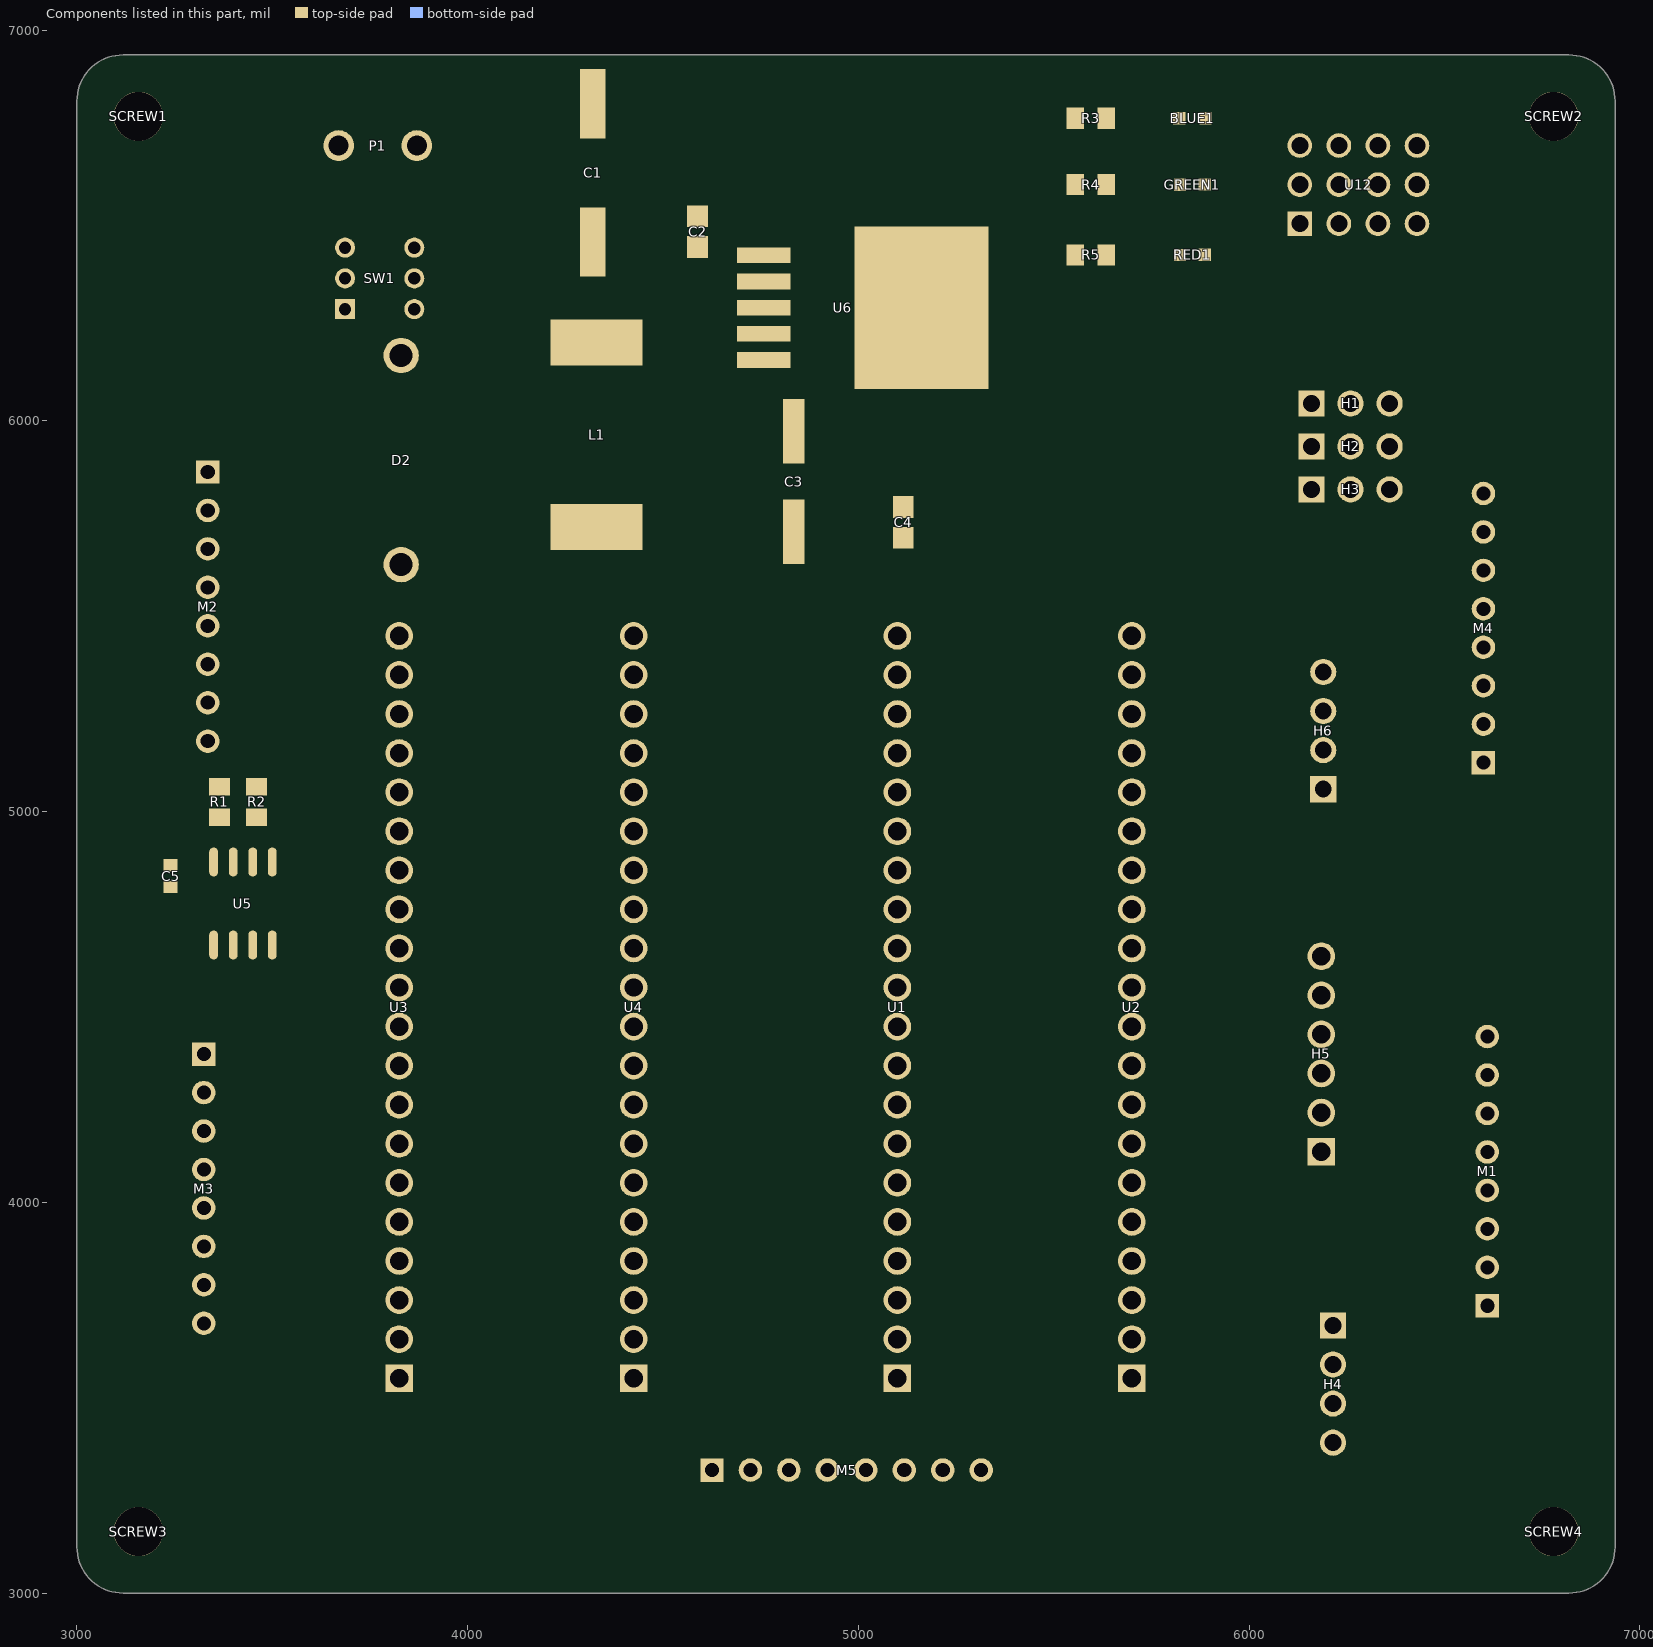
[diagram p0: the components of this part, seen from the top]
# Altium PCB MISC50151.pcbdoc (part 4 of 4)
Units mil, origin at the board's own origin, x right, y up, seen from the top; angles counter-clockwise.
Board outline 3937.01 x 3937.01 mil, 4 copper layers (Top Layer, Inner1, Inner2, Bottom Layer), stack 62.447 mil thick; 39 components, 26 nets, 211 pads, 230 vias.

## Other copper (continued)
Bottom Layer:
  region net M_PWM1: 6324.25,6073.68 6331.32,6080.75 6334.09,6080.42 6341.11,6079.85 6362.1,6078.4 6326.6,6042.9 6325.15,6063.89 6324.58,6070.91
  region net M_PWM2: 6388.68,5970.75 6395.75,5963.68 6395.42,5960.91 6394.85,5953.89 6393.4,5932.9 6357.9,5968.4 6378.89,5969.85 6385.91,5970.42
  region net M_PWM3: 6365,5779.44 6355,5779.44 6353.27,5781.63 6348.72,5787 6334.9,5802.87 6385.1,5802.87 6371.28,5787 6366.73,5781.63
  region net M_PWM3: 5748.24,3955 5748.24,3945 5740.36,3938.26 5723.44,3923.43 5723.44,3976.57 5740.36,3961.74
  region net M_MASTER_TX: 5741,4085.56 5738.69,4069.1 5737.49,4067.67 5736.53,4066.03 5735.78,4064.21 5735.21,4062.25 5734.8,4060.18 5734.52,4058.03 5734.26,4053.6 5734.28,4045.18 5734.16,4041.69 5733.98,4040.23 5733.69,4039.02 5706.68,4084.8 5712.07,4083.93 5717.55,4083.34 5722.91,4083.04 5727.96,4083.01 5732.5,4083.25 5736.32,4083.76 5739.22,4084.53 5740.26,4085.01
  region net M_MASTER_RX: 5734.87,4186.94 5738.19,4176.12 5737.01,4174.67 5736.08,4172.99 5735.37,4171.11 5734.87,4169.07 5734.54,4166.89 5734.36,4164.62 5734.34,4159.93 5734.59,4155.27 5734.92,4150.92 5735.11,4147.16 5734.97,4144.26 5701.32,4185.41 5712.89,4185.22 5723.38,4185.45 5731.23,4186.05 5733.67,4186.46
  region net M_GYRO_SCL: 5748.24,4855 5748.24,4845 5740.36,4838.26 5723.44,4823.43 5723.44,4876.57 5740.36,4861.74
  region net M_GYRO_SDA: 5748.24,4955 5748.24,4945 5740.36,4938.26 5723.44,4923.43 5723.44,4976.57 5740.36,4961.74
  region net M_PWM1: 5130.58,4387.65 5137.65,4380.58 5136.84,4370.24 5135.36,4347.78 5097.78,4385.36 5120.24,4386.84
  region net M_PWM2: 5130.58,4487.65 5137.65,4480.58 5136.84,4470.24 5135.36,4447.78 5097.78,4485.36 5120.24,4486.84
  region net 12.6V: 6624.7,5171.42 6645.91,5150.21 6641.8,5144.16 6638.26,5137.77 6635.32,5131.07 6633.01,5124.14 6631.34,5117.02 6630.34,5109.78 6630,5102.48 6576.97,5155.51 6584.27,5155.85 6591.51,5156.85 6598.63,5158.52 6605.56,5160.83 6612.26,5163.77 6618.65,5167.31 6624.7,5171.42
  region net M_MASTER_RX: 6154.42,4592.35 6147.35,4599.42 6148.16,4609.76 6149.64,4632.22 6187.22,4594.64 6164.76,4593.16
  region net M_MASTER_TX: 6154.42,4492.35 6147.35,4499.42 6148.16,4509.76 6149.64,4532.22 6187.22,4494.64 6164.76,4493.16
  region net M_GYRO_SCL: 6144.44,5252.57 6144.44,5262.57 6146.63,5264.29 6152,5268.85 6167.87,5282.67 6167.87,5232.47 6152,5246.29 6146.63,5250.84
  region net M_GYRO_SDA: 6144.44,5352.57 6144.44,5362.57 6146.63,5364.29 6152,5368.85 6167.87,5382.67 6167.87,5332.47 6152,5346.29 6146.63,5350.84

## Silkscreen, mask and mechanical layers (free items; w line width, h text height)
Top Silkscreen Layer:
  lines w10: 6235,4482.56 6235,4680 6460.79,4680 6460.79,4482.56 6235,4482.56 ; 6235,4482.56 6460,4482.56 6460,4080 6235,4080 6235,4482.56 ; 3675,3450 3675,5550 4575,5550 4575,3450 3675,3450 ; 4950,3450 4950,5550 5850,5550 5850,3450 4950,3450
  text "5V" at 6505,6675 h80
  text "3.3V" at 6500,6570 h80
  text "GND" at 6495,6465 h80
  text "5V" at 6295,6125 h80 r90
  text "GND" at 6195,6119.88 h80 r90
  text "TIM1" at 6400,6120 h80 r90
  text "CH1" at 5970,6010.21 h80
  text "CH2" at 5969.88,5890.21 h80
  text "CH3" at 5969.88,5780.21 h80
  text "I2C1" at 6132.3,5425 h60
  text "Master" at 5274.61,5405 h120
  text "Slave" at 3999.07,5390 h120
  text "SDA" at 6255,5325 h60
  text "SCL" at 6255,5230 h60
  text "OLED" at 6105,5145 h80 r90
  text "3.3V" at 6254.55,5125 h60
  text "GND" at 6255,5030 h60
  text "M_1_RX" at 6245,4600 h60
  text "M_1_TX" at 6245,4500 h60
  text "M_2_RX" at 6245,4395 h60
  text "S_2_TX" at 6245,4300 h60
  text "S_3_RX" at 6245,4200 h60
  text "Reserved & host PC" at 6115,4115 h80 r90
  text "S_3_TX" at 6245,4100 h60
  text "I2C2" at 6155,3750 h60
  text "5V" at 6289.42,3660 h60
  text "SCL" at 6289.88,3555 h60
  text "SDA" at 6289.88,3455 h60
  text "Gyroscope" at 6135,3410 h80 r90
  text "GND" at 6289.88,3350 h60